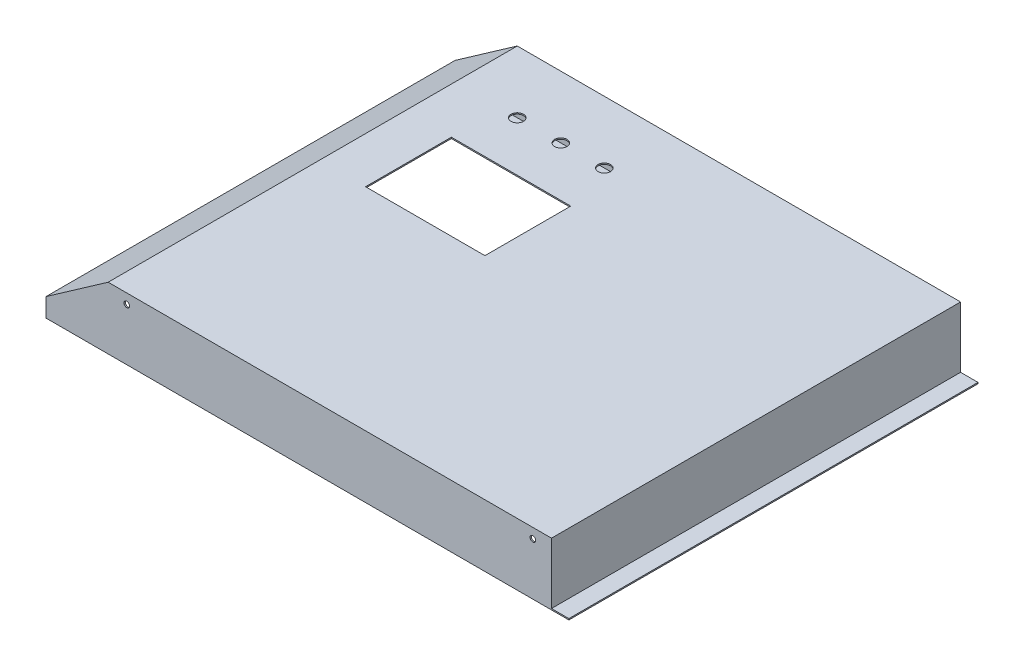
SolidWorks part; units mm, degrees
ref_plane "前视" through (0, 0, 0) normal (0, 0, 1) x (1, 0, 0)
ref_plane "上视" through (0, 0, 0) normal (0, 1, 0) x (1, 0, 0)
ref_plane "右视" through (0, 0, 0) normal (1, 0, 0) x (0, 0, -1)
sketch "草图1" plane through (0, 0, 0) normal (0, 0, 1) x (1, 0, 0)
  line L0 (0, 0) -> (0, 34.8107) construction
  line L1 (0, 0) -> (56.1399, 0) construction
  line L2 (0, 0) -> (-813, 0)
  line L3 (-813, 0) -> (-813, 30)
  line L4 (0, 0) -> (0, 100)
  line L5 (0, 100) -> (-713.0296, 100)
  line L6 (-713.0296, 100) -> (-813, 30)
  line L7 (0, 0) -> (0, 353.3141) construction
  dimension "D1" = 813
  dimension "D2" = 30
  dimension "D3" = 145
  dimension "D4" = 100
extrude "凸台-拉伸1" add sketch "草图1" along normal mid plane 658
shell "抽壳1" thickness 2
sketch "草图2" plane through (0, 100, 0) normal (0, 1, 0) x (1, 0, 0)
  line L0 (0, 329) -> (-713.0296, 329) construction
  line L1 (-639.0296, 149) -> (-447.0296, 149)
  line L2 (-639.0296, 149) -> (-639.0296, 11)
  line L3 (-639.0296, 11) -> (-447.0296, 11)
  line L4 (-447.0296, 149) -> (-447.0296, 11)
  line L5 (-713.0296, -329) -> (-713.0296, 329) construction
  line L6 (-543.0296, 149) -> (-543.0296, 365.9839) construction
  circle A0 centre (-613.0296, 229) radius 10
  circle A1 centre (-543.0296, 229) radius 10
  circle A2 centre (-473.0296, 229) radius 10
  dimension "D5" = 70
  dimension "D1" = 138
  dimension "D2" = 192
  dimension "D3" = 180
  dimension "D4" = 74
  dimension "D6" = 80
  dimension "D7" = 80
extrude "切除-拉伸1" cut sketch "草图2" against normal blind 658
sketch "草图3" plane through (0, 0, 0) normal (0, -1, 0) x (1, 0, 0)
  line L0 (-813, 329) -> (0, 329) construction
  line L1 (-2, 329) -> (28, 329)
  line L2 (-2, 329) -> (-2, -329)
  line L3 (-2, -329) -> (28, -329)
  line L4 (28, 329) -> (28, -329)
  line L5 (-2, 327) -> (-2, -327) construction
  dimension "D1" = 30
extrude "凸台-拉伸2" add sketch "草图3" against normal blind 2
sketch "草图4" plane through (0, 0, 0) normal (0, -1, 0) x (1, 0, 0)
  line L0 (-783, 299) -> (-783, -299)
  line L1 (-813, 329) -> (0, 329)
  line L2 (-813, 329) -> (-813, -329)
  line L3 (-813, -329) -> (0, -329)
  line L4 (0, 329) -> (0, 299)
  line L5 (-783, 299) -> (0, 299)
  line L6 (-783, -299) -> (0, -299)
  line L7 (0, -299) -> (0, -329)
  line L8 (-30, 299) -> (-30, -299) construction
  line L9 (-783, 299) -> (-30, 299) construction
  line L10 (-783, -299) -> (-30, -299) construction
  line L12 (0, 329) -> (0, -329) construction
  dimension "D1" = 30
extrude "凸台-拉伸3" add sketch "草图4" against normal blind 2
sketch "草图5" plane through (0, 0, 329) normal (0, 0, 1) x (1, 0, 0)
  line L2 (0, 84) -> (-713.0296, 84)
  line L3 (0, 84) -> (-713.0296, 84) construction
  line L4 (-713.0296, 100) -> (-713.0296, -59.8184) construction
  line L5 (-30, 2) -> (-30, 100)
  line L6 (-30, 2) -> (-30, 100) construction
  line L7 (-683.0296, 100) -> (-683.0296, -59.8184) construction
  circle A0 centre (-683.0296, 84) radius 4.5
  circle A1 centre (-30, 84) radius 4.5
  dimension "D4" = 9
  dimension "D5" = 9
  dimension "D1" = 16
  dimension "D2" = 30
  dimension "D3" = 30
extrude "切除-拉伸2" cut sketch "草图5" against normal blind 797
sketch "草图6" plane through (0, 0, 0) normal (0, -1, 0) x (1, 0, 0)
  line L6 (-797, 0) -> (-941.5015, 0) construction
  line L7 (-813, -329) -> (28, -329) construction
  line L8 (-813, 329) -> (28, 329) construction
  line L9 (-2, -313) -> (-797, -313)
  line L10 (-797, 313) -> (-2, 313)
  line L11 (-797, -313) -> (-797, 313)
  line L12 (-2, -313) -> (-797, -313) construction
  line L13 (-797, 313) -> (-2, 313) construction
  line L14 (-797, -313) -> (-797, 313) construction
  circle A0 centre (-797, 299) radius 4.5
  circle A1 centre (-797, -299) radius 4.5
  circle A2 centre (-797, 0) radius 4.5
  dimension "D2" = 9
  dimension "D3" = 9
  dimension "D4" = 30
  dimension "D5" = 30
  dimension "D6" = 9
  dimension "D1" = 14
extrude "切除-拉伸3" cut sketch "草图6" against normal blind 10
